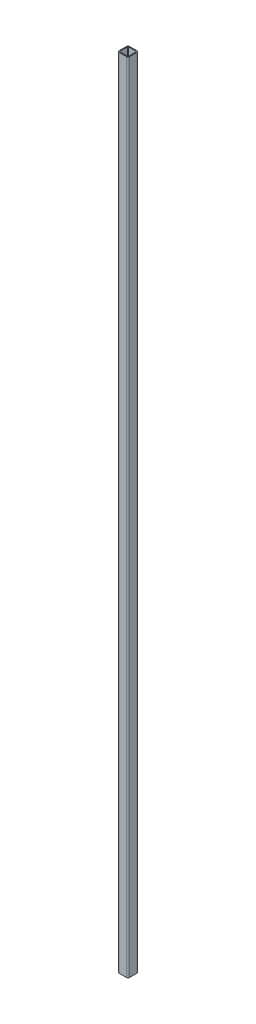
from build123d import *

# Parameters (mm, degrees)
COLD_FORMED_HOLLOW_SQUARE_STEEL_GB_T_67_DEPTH = 9220


with BuildPart() as part:
    # Sketch12 → Cold-formed hollow square steel (GB/T 6728-2002) 120×120×10(1) (new body)
    with BuildSketch(Plane(origin=(0, 0, 0), x_dir=(-1, 0, 0), z_dir=(0, 1, 0))):
        with BuildLine():
            Line((-44, -60), (44, -60))
            ThreePointArc((44, -60), (55.313708499, -55.313708499), (60, -44))
            Line((60, -44), (60, 44))
            ThreePointArc((60, 44), (55.313708499, 55.313708499), (44, 60))
            Line((44, 60), (-44, 60))
            ThreePointArc((-44, 60), (-55.313708499, 55.313708499), (-60, 44))
            Line((-60, 44), (-60, -44))
            ThreePointArc((-60, -44), (-55.313708499, -55.313708499), (-44, -60))
        make_face()
        with BuildLine():
            Line((-44, -50), (44, -50))
            ThreePointArc((44, -50), (48.242640687, -48.242640687), (50, -44))
            Line((50, -44), (50, 44))
            ThreePointArc((50, 44), (48.242640687, 48.242640687), (44, 50))
            Line((44, 50), (-44, 50))
            ThreePointArc((-44, 50), (-48.242640687, 48.242640687), (-50, 44))
            Line((-50, 44), (-50, -44))
            ThreePointArc((-50, -44), (-48.242640687, -48.242640687), (-44, -50))
        make_face(mode=Mode.SUBTRACT)
    extrude(amount=COLD_FORMED_HOLLOW_SQUARE_STEEL_GB_T_67_DEPTH)


solid = part.part
